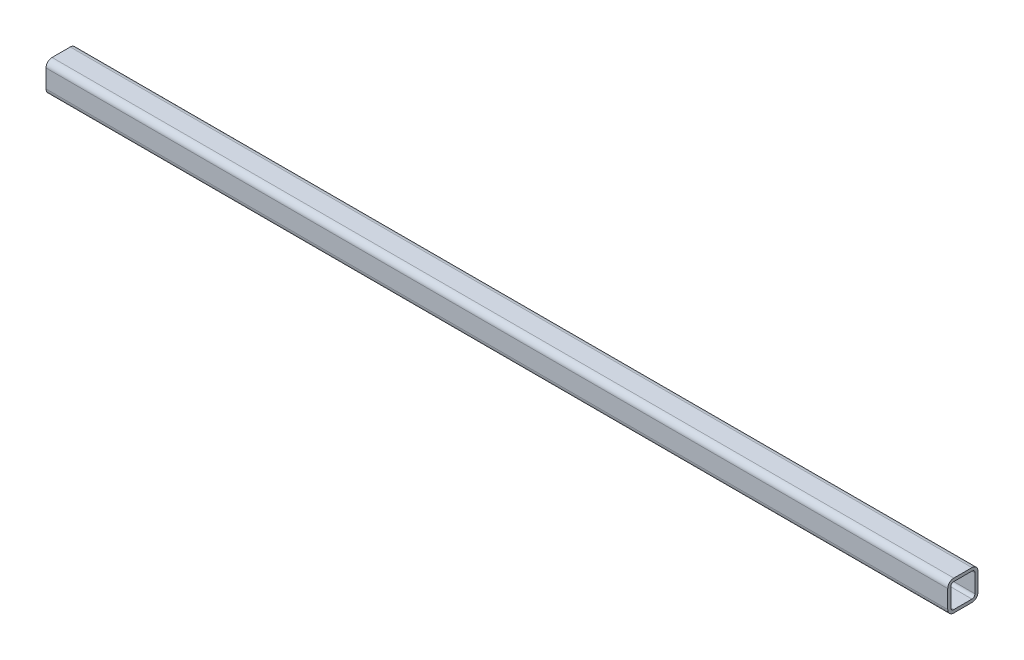
SolidWorks part; units mm, degrees
material "普通碳钢"
ref_plane "Front Plane" through (0, 0, 0) normal (0, 0, 1) x (1, 0, 0)
ref_plane "Top Plane" through (0, 0, 0) normal (0, 1, 0) x (1, 0, 0)
ref_plane "Right Plane" through (0, 0, 0) normal (1, 0, 0) x (0, 0, -1)
sketch "草图1" plane through (0, 0, 0) normal (0, 0, 1) x (1, 0, 0)
  line L0 (-1000, 0) -> (192, 0)
  dimension "D1" = 1192
  dimension "D2" = 1000
other "Square Tube 40 X 40 X 4(1)"
ref_plane "Plane1" through (-1000, 0, 0) normal (1, 0, 0) x (0, 1, 0)
sketch "Sketch1" plane through (-1000, 0, 0) normal (1, 0, 0) x (0, 1, 0)
  line L0 (-12, -16) -> (12, -16)
  line L1 (-16, -12) -> (-16, 12)
  line L2 (12, 16) -> (-12, 16)
  line L3 (16, 12) -> (16, -12)
  line L4 (-12, -20) -> (12, -20)
  line L5 (-20, -12) -> (-20, 12)
  line L6 (12, 20) -> (-12, 20)
  line L7 (20, 12) -> (20, -12)
  arc A0 (20, 12) -> (12, 20) centre (12, 12) ccw
  arc A1 (12, -20) -> (20, -12) centre (12, -12) ccw
  arc A2 (-20, -12) -> (-12, -20) centre (-12, -12) ccw
  arc A3 (-12, 20) -> (-20, 12) centre (-12, 12) ccw
  arc A4 (-12, 16) -> (-16, 12) centre (-12, 12) ccw
  arc A5 (16, 12) -> (12, 16) centre (12, 12) ccw
  arc A6 (12, -16) -> (16, -12) centre (12, -12) ccw
  arc A7 (-16, -12) -> (-12, -16) centre (-12, -12) ccw
  point P0 (-20, 0)
  point P1 (20, 0)
  point P2 (0, 20)
  point P3 (0, -20)
  point P4 (0, 0)
  point P5 (-20, -20)
  point P6 (20, -20)
  point P7 (20, 20)
  point P8 (-20, 20)
  point P33 (0, 0)
  dimension "D1" = 8
  dimension "Thickness" = 4
  dimension "V_leg" = 40
